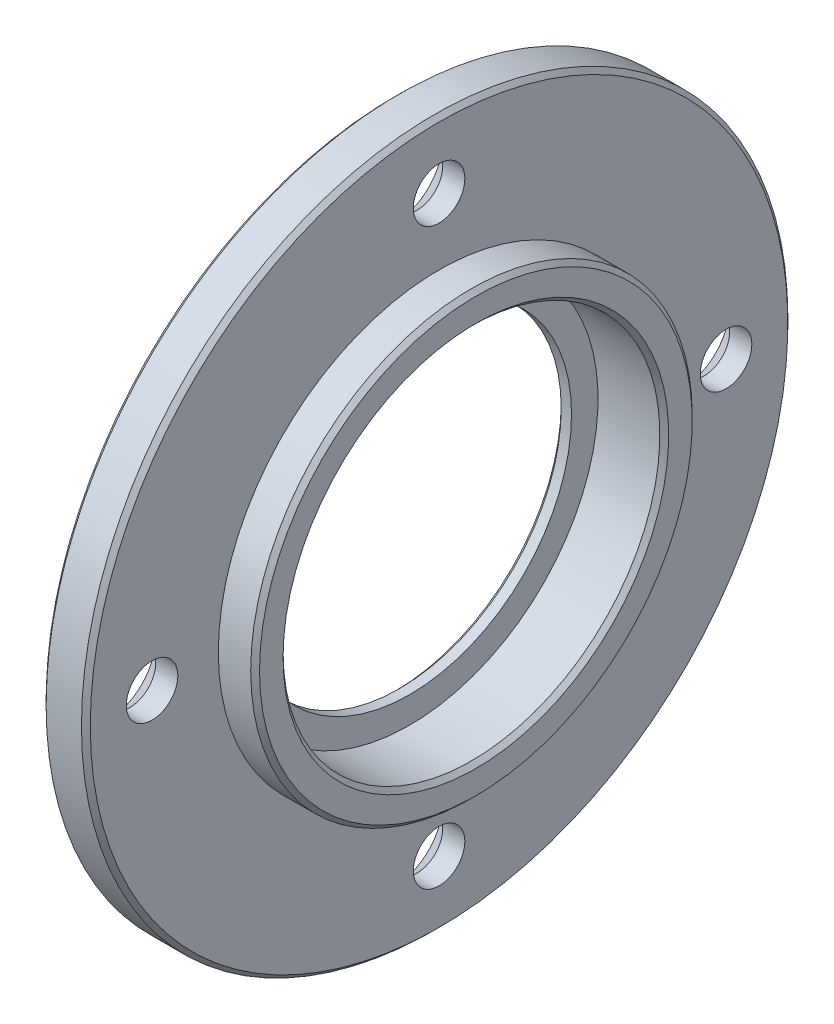
SolidWorks part; units mm, degrees
ref_plane "Front Plane" through (0, 0, 0) normal (0, 0, 1) x (1, 0, 0)
ref_plane "Top Plane" through (0, 0, 0) normal (0, 1, 0) x (1, 0, 0)
ref_plane "Right Plane" through (0, 0, 0) normal (1, 0, 0) x (0, 0, -1)
sketch "Sketch1" plane through (0, 0, 0) normal (0, 0, 1) x (1, 0, 0)
  line L0 (0, 11) -> (0, 24)
  line L4 (5.5, 15) -> (5.5, 12.8)
  line L5 (5.5, 12.8) -> (1, 12.8)
  line L6 (1, 12.8) -> (1, 11)
  line L7 (1, 11) -> (0, 11)
  line L8 (0, 0) -> (73.7918, 0) construction
  line L9 (3, 24) -> (0, 24)
  line L10 (5.5, 15) -> (3, 15)
  line L11 (3, 15) -> (3, 24)
  dimension "D1" = 12.8
  dimension "D2" = 4.5
  dimension "D3" = 1
  dimension "D4" = 11
  dimension "D5" = 3
  dimension "D6" = 15
  dimension "D7" = 24
revolve "Revolve1" add sketch "Sketch1" angle 360 about L8
sketch "Sketch2" plane through (3, 0, 0) normal (1, 0, 0) x (0, 0, -1)
  circle A0 centre (0, 0) radius 19.5 construction
  circle A1 centre (0, 19.5) radius 1.75
  circle A2 centre (19.5, 0) radius 1.75
  circle A3 centre (0, -19.5) radius 1.75
  circle A4 centre (-19.5, 0) radius 1.75
  dimension "D1" = 39
  dimension "D2" = 3.5
extrude "Cut-Extrude1" cut sketch "Sketch2" against normal up to surface (3 mm away) up to face at (0, 0, 11)
chamfer "Chamfer1" distance 1.5 angle 45 4 edges at (0, 0, 17.75) (0, -19.5, -1.75) (0, 19.5, -1.75) (0, 0, -21.25)
chamfer "Chamfer2" distance 0.3 angle 45 5 edges at (5.5, 0, 15) (5.5, 0, 12.8) (3, 0, 24) (0, 0, 24) (0, 0, 11)
